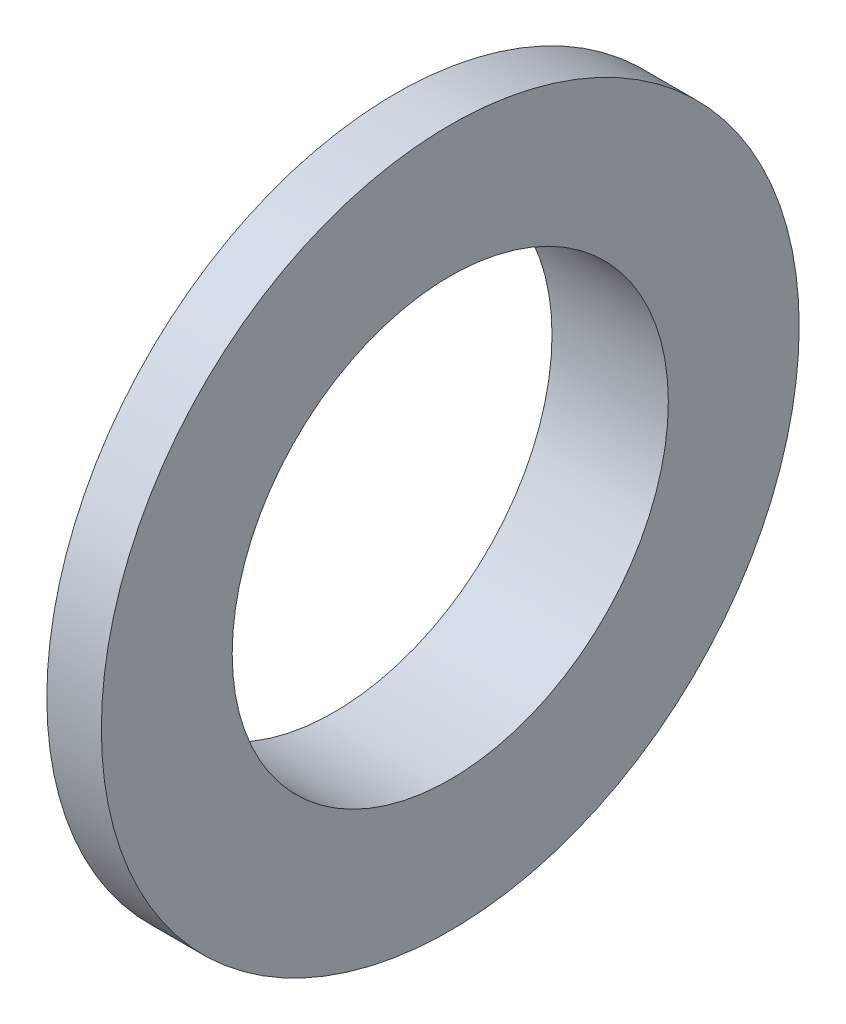
from build123d import *


with BuildPart() as part:
    # Sketch1 → Revolve1 (revolve)
    with BuildSketch(Plane.XY, mode=Mode.PRIVATE) as revolve1_sk:
        Polygon((0, 120), (0, 140), (48, 140), (48, 154), (34, 154), (34, 166), (48, 166), (48, 180), (34, 180), (34, 192), (64, 192), (64, 120), align=None)
    revolve(revolve1_sk.sketch.rotate(Axis((0, 0, 0), (1, 0, 0)), 90), axis=Axis((0, 0, 0), (1, 0, 0)))


solid = part.part
